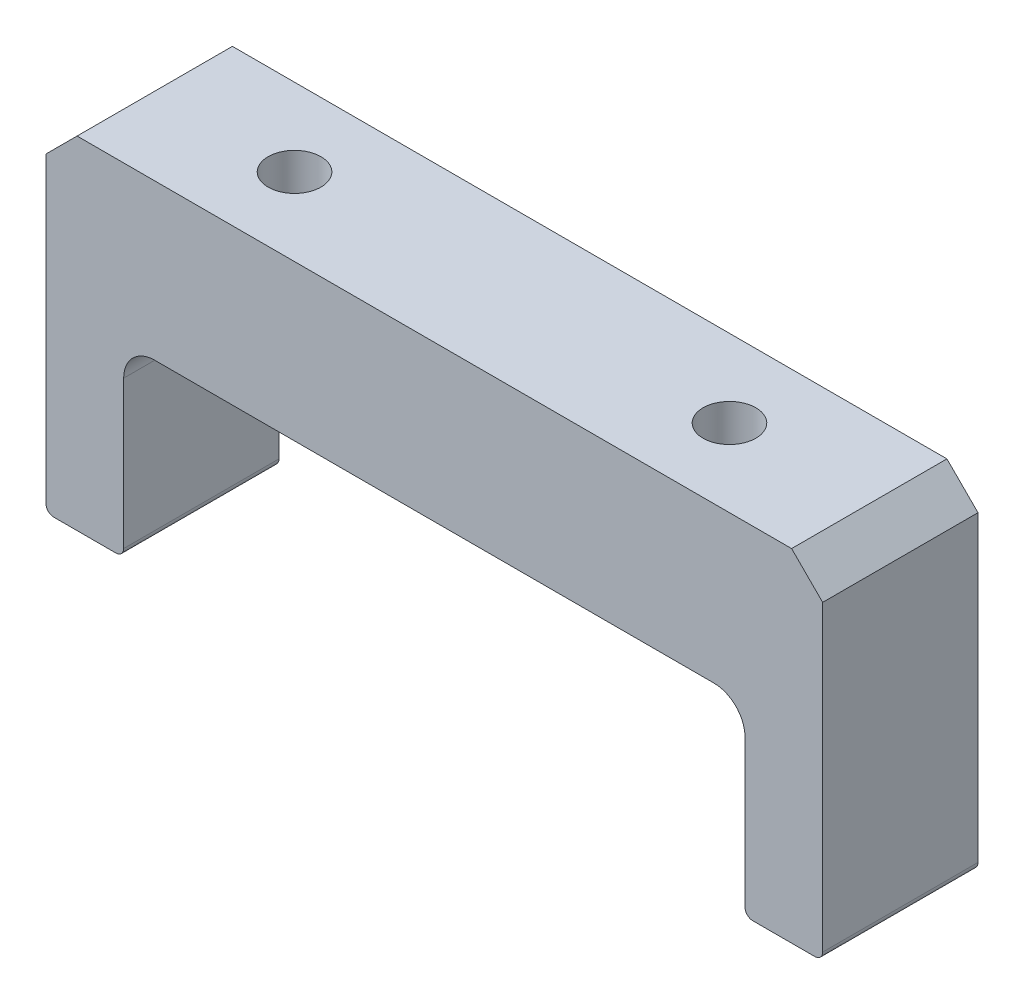
from build123d import *

# Parameters (mm, degrees)
BOSS_EXTRUDE1_DEPTH                     = 10
CBORE_FOR_M3_HEX_HEAD_BOLT1_D           = 3.4
CBORE_FOR_M3_HEX_HEAD_BOLT1_CBORE_D     = 6
CBORE_FOR_M3_HEX_HEAD_BOLT1_CBORE_DEPTH = 3.5
FILLET1_R                               = 2
FILLET2_R                               = 0.5
CHAMFER1_SIZE                           = 2


with BuildPart() as part:
    # Sketch1 → Boss-Extrude1 (new body)
    with BuildSketch(Plane.XY):
        Polygon((45, -22), (50, -22), (50, 0), (0, 0), (0, -22), (5, -22), (5, -10), (45, -10), align=None)
    extrude(amount=BOSS_EXTRUDE1_DEPTH)

    # CBORE for M3 Hex Head Bolt1 (through all)
    with Locations(Plane.XZ.offset(10)):
        with Locations((11, 5), (39, 5)):
            CounterBoreHole(CBORE_FOR_M3_HEX_HEAD_BOLT1_D / 2, CBORE_FOR_M3_HEX_HEAD_BOLT1_CBORE_D / 2, CBORE_FOR_M3_HEX_HEAD_BOLT1_CBORE_DEPTH)

    # Fillet1
    fillet1_edges = [part.edges().sort_by_distance(p)[0] for p in [
        (45, -10, 5),
        (5, -10, 5),
    ]]
    fillet(fillet1_edges, radius=FILLET1_R)

    # Fillet2
    fillet2_edges = [part.edges().sort_by_distance(p)[0] for p in [
        (50, -22, 5),
        (45, -22, 5),
        (5, -22, 5),
        (0, -22, 5),
    ]]
    fillet(fillet2_edges, radius=FILLET2_R)

    # Chamfer1
    chamfer1_edges = [part.edges().sort_by_distance(p)[0] for p in [
        (0, 0, 5),
        (50, 0, 5),
    ]]
    chamfer(chamfer1_edges, length=CHAMFER1_SIZE)


solid = part.part
